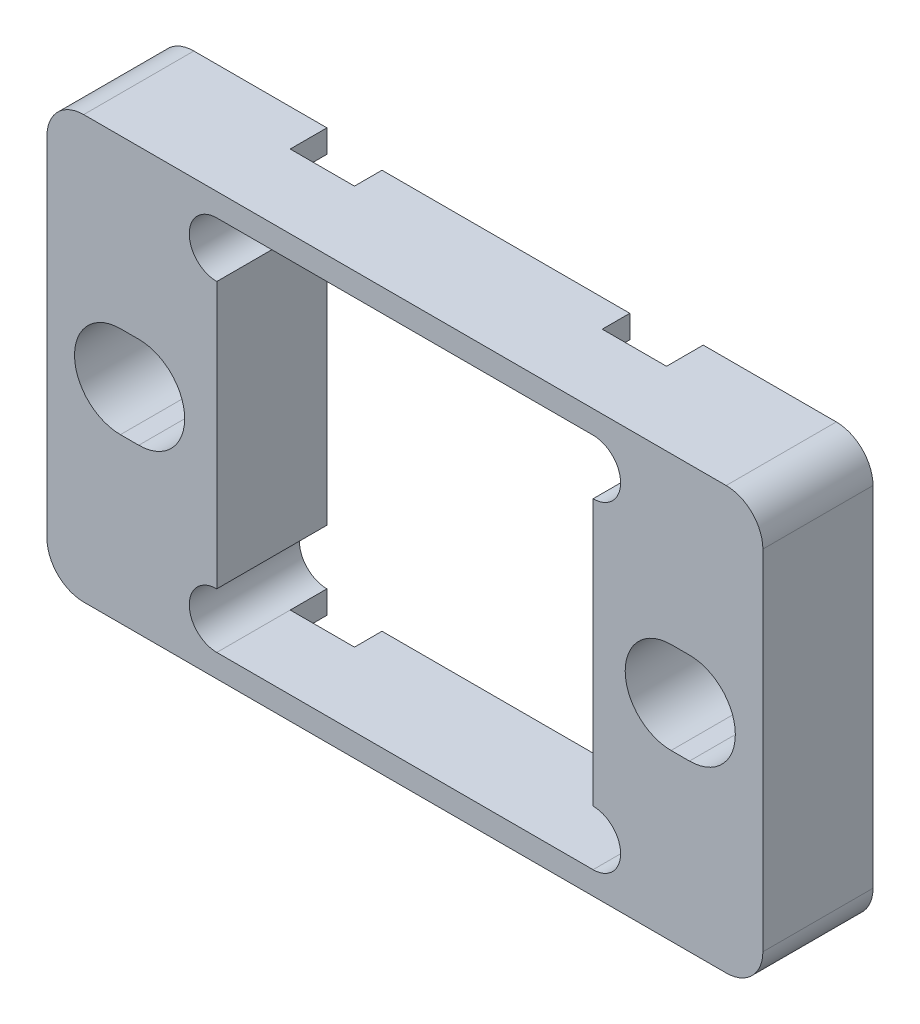
SolidWorks part; units mm, degrees
ref_plane "Front Plane" through (0, 0, 0) normal (0, 0, 1) x (1, 0, 0)
ref_plane "Top Plane" through (0, 0, 0) normal (0, 1, 0) x (1, 0, 0)
ref_plane "Right Plane" through (0, 0, 0) normal (1, 0, 0) x (0, 0, -1)
sketch "Sketch1" plane through (0, 0, 0) normal (0, 0, 1) x (1, 0, 0)
  line L1 (-19.5, 11.5) -> (19.5, 11.5)
  line L2 (-19.5, 11.5) -> (-19.5, -11.5)
  line L3 (-19.5, -11.5) -> (19.5, -11.5)
  line L4 (19.5, 11.5) -> (19.5, -11.5)
  line L5 (-19.5, 11.5) -> (19.5, -11.5) construction
  line L6 (-19.5, -11.5) -> (19.5, 11.5) construction
  line L7 (-10.25, 10.25) -> (10.25, 10.25)
  line L8 (-10.25, 10.25) -> (-10.25, -10.25)
  line L9 (-10.25, -10.25) -> (10.25, -10.25)
  line L10 (10.25, 10.25) -> (10.25, -10.25)
  line L11 (-10.25, 10.25) -> (10.25, -10.25) construction
  line L12 (-10.25, -10.25) -> (10.25, 10.25) construction
  point P0 (0, 0)
  point P5 (0, 0)
  dimension "D1" = 23
  dimension "D2" = 39
  dimension "D3" = 20.5
extrude "Boss-Extrude1" add sketch "Sketch1" along normal blind 6
sketch "Sketch2" plane through (0, -11.5, 0) normal (0, -1, 0) x (1, 0, 0)
  line L0 (0, 0) -> (0, 6) construction
  line L1 (-19.5, 6) -> (19.5, 6) construction
  line L2 (-19.5, 0) -> (19.5, 0) construction
  line L3 (-10.25, 6) -> (10.25, 6)
  line L4 (-10.25, 6) -> (-10.25, 1.65)
  line L5 (-10.25, 1.65) -> (10.25, 1.65)
  line L6 (10.25, 6) -> (10.25, 1.65)
  dimension "D1" = 20.5
  dimension "D2" = 1.65
extrude "Cut-Extrude1" cut sketch "Sketch2" against normal up to surface (23 mm away) up to face at (0, 11.5, 3)
sketch "Sketch3" plane through (0, 0, 6) normal (0, 0, 1) x (1, 0, 0)
  line L1 (-10.25, 11.5) -> (10.25, 11.5)
  line L2 (-10.25, 11.5) -> (-10.25, 10.25)
  line L3 (-10.25, 10.25) -> (10.25, 10.25)
  line L4 (10.25, 11.5) -> (10.25, 10.25)
  line L5 (-10.25, -10.25) -> (10.25, -10.25)
  line L6 (-10.25, -10.25) -> (-10.25, -11.5)
  line L7 (-10.25, -11.5) -> (10.25, -11.5)
  line L8 (10.25, -10.25) -> (10.25, -11.5)
extrude "Boss-Extrude2" add sketch "Sketch3" against normal up to surface (4.35 mm away) up to face at (0, -10.875, 1.65)
sketch "Sketch4" plane through (0, -11.5, 0) normal (0, -1, 0) x (1, 0, 0)
  line L0 (0, 0) -> (0, 6) construction
  line L1 (-19.5, 6) -> (19.5, 6) construction
  line L2 (6.75, 0.5) -> (6.75, 2)
  line L3 (-10.25, 0) -> (-6.75, 0)
  line L4 (-10.25, 0) -> (-10.25, 2)
  line L5 (-10.25, 2) -> (-6.75, 2)
  line L6 (-6.75, 0.5) -> (-6.75, 2)
  line L7 (10.25, 2) -> (6.75, 2)
  line L8 (10.25, 0) -> (10.25, 2)
  line L9 (10.25, 0) -> (6.75, 0)
  line L11 (-6.75, 0) -> (6.75, 0)
  line L13 (-6.75, 0.5) -> (6.75, 0.5)
  dimension "D1" = 3.5
  dimension "D2" = 2
  dimension "D3" = 0.5
extrude "Cut-Extrude2" cut sketch "Sketch4" against normal up to surface (23 mm away) up to face at (0, 11.5, 3)
sketch "Sketch5" plane through (0, 0, 0) normal (0, 0, -1) x (-1, 0, 0)
  line L0 (-10.25, 8.75) -> (10.25, 8.75) construction
  line L1 (-10.25, -11.5) -> (-10.25, 11.5) construction
  line L2 (10.25, 11.5) -> (10.25, -11.5) construction
  line L3 (-10.25, 10.25) -> (10.25, 10.25)
  line L4 (-10.25, 7.25) -> (10.25, 7.25)
  line L5 (-10.25, -8.75) -> (10.25, -8.75) construction
  line L6 (-10.25, -7.25) -> (10.25, -7.25)
  line L7 (-10.25, -10.25) -> (10.25, -10.25)
  line L8 (-10.25, 10.25) -> (-6.75, 10.25) construction
  line L9 (-6.75, -10.25) -> (-10.25, -10.25) construction
  arc A0 (-10.25, 10.25) -> (-10.25, 7.25) centre (-10.25, 8.75) ccw
  arc A1 (10.25, 7.25) -> (10.25, 10.25) centre (10.25, 8.75) ccw
  arc A2 (-10.25, -7.25) -> (-10.25, -10.25) centre (-10.25, -8.75) ccw
  arc A3 (10.25, -10.25) -> (10.25, -7.25) centre (10.25, -8.75) ccw
  point P6 (0, 8.75)
  point P11 (0, -8.75)
  dimension "D1" = 1.5
extrude "Cut-Extrude3" cut sketch "Sketch5" against normal up to surface (6 mm away)
sketch "Sketch6" plane through (0, 0, 6) normal (0, 0, 1) x (1, 0, 0)
  line L0 (-15.5, -0.1) -> (-14.5, -0.1) construction
  line L1 (-15.5, 2.4) -> (-14.5, 2.4)
  line L2 (-15.5, -2.6) -> (-14.5, -2.6)
  line L3 (14.5, 0) -> (15.5, 0) construction
  line L4 (14.5, 2.5) -> (15.5, 2.5)
  line L5 (14.5, -2.5) -> (15.5, -2.5)
  arc A0 (-15.5, 2.4) -> (-15.5, -2.6) centre (-15.5, -0.1) ccw
  arc A1 (-14.5, -2.6) -> (-14.5, 2.4) centre (-14.5, -0.1) ccw
  arc A2 (14.5, 2.5) -> (14.5, -2.5) centre (14.5, 0) ccw
  arc A3 (15.5, -2.5) -> (15.5, 2.5) centre (15.5, 0) ccw
  point P4 (-15, -0.1)
  point P9 (15, 0)
  dimension "D1" = 2.5
extrude "Cut-Extrude4" cut sketch "Sketch6" against normal blind 10
fillet "Fillet1" radius 2 4 edges at (-19.5, 11.5, 3) (-19.5, -11.5, 3) (19.5, -11.5, 3) (19.5, 11.5, 3)
